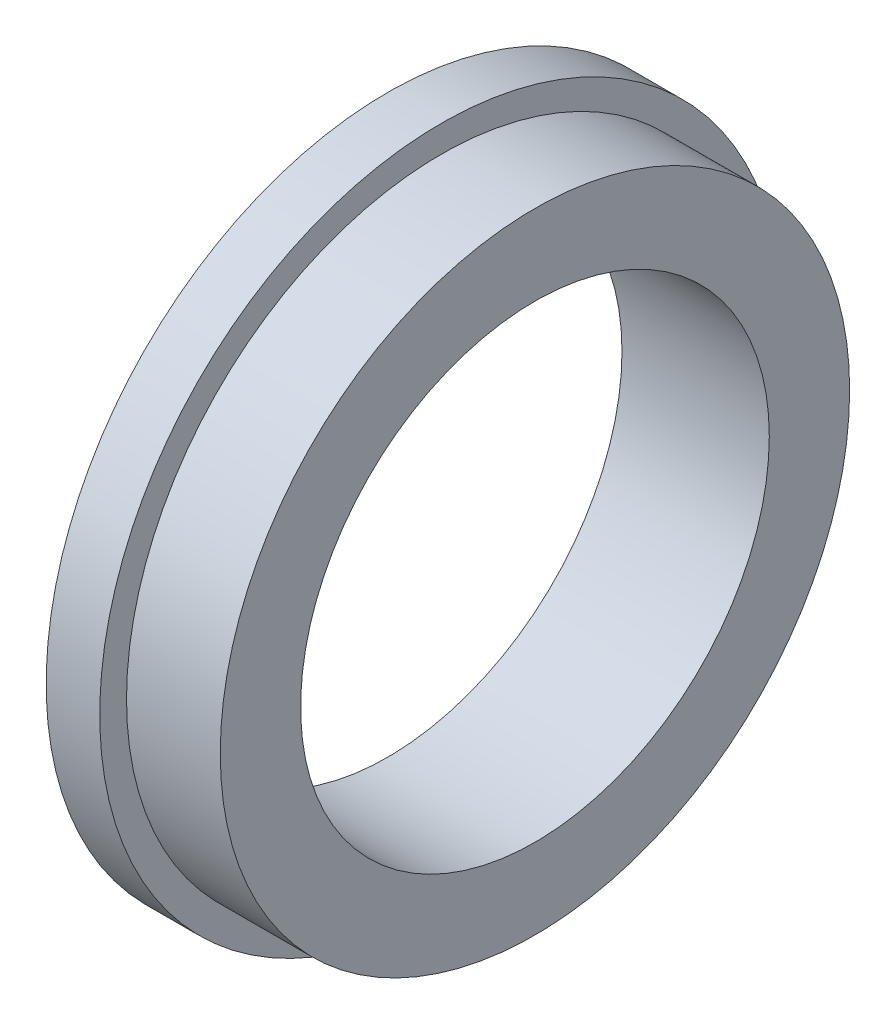
from build123d import *

# Parameters (mm, degrees)
SCALE_1_SCALE = 1.875


with BuildPart() as part:
    # Sketch1 → Revolve1 (revolve)
    with BuildSketch(Plane.XY, mode=Mode.PRIVATE) as revolve1_sk:
        Polygon((-7.228973684, 17.5), (3.771026316, 17.5), (3.771026316, 23.5), (-3.228973684, 23.5), (-3.228973684, 25.5), (-7.228973684, 25.5), align=None)
    revolve(revolve1_sk.sketch.rotate(Axis((0, 0, 0), (-1, 0, 0)), 90), axis=Axis((0, 0, 0), (-1, 0, 0)))


with BuildPart() as part_1:
    # Scale 1: scaled about (-2.17184005, 0, 0)
    add(part.part.scale(SCALE_1_SCALE).moved(Location((1.900360044, 0, 0))))


solid = part_1.part
